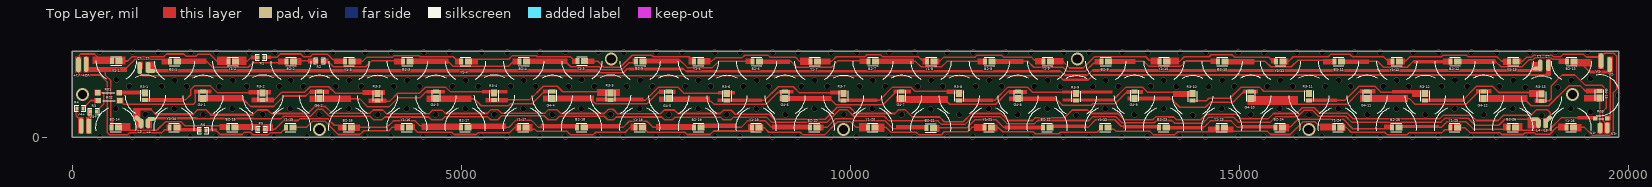
[diagram p0: Top Layer view]
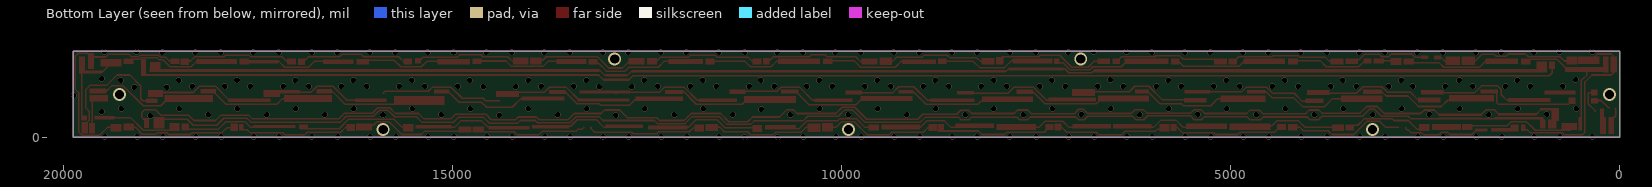
[diagram p1: Bottom Layer view, seen from below]
# Altium PCB MISC59163.PcbDoc
Units mil, origin at the board's own origin, x right, y up, seen from the top; angles counter-clockwise.
Board outline 19875 x 1102.36 mil, 2 copper layers (Top Layer, Bottom Layer); 87 components, 89 nets, 196 pads, 241 vias.

## Layer stack, top to bottom (the 12.6 mil dielectric is the usual default, probably not edited)
Top Solder: solder mask 0.4, Solder Resist, Dk 3.5
Top Layer: signal copper 1.4
Dielectric 1: dielectric 12.6, FR-4, Dk 4.8
Bottom Layer: signal copper 1.4
Bottom Solder: solder mask 0.4, Solder Resist, Dk 3.5

## Board outline
0,0 19875,0 19875,1102.36 0,1102.36

## Design rules (kind name [scope] priority, off if disabled: settings)
Clearance [All] p1: gap=0 ignorepadtopadclearanceinfootprint=TRUE
ComponentClearance [All] p1: gap=0 collisioncheckmode=3 verticalgap=0 showdistances=FALSE
HoleSize [All] p1: absolutevalues=TRUE maxlimit=1000 minlimit=1 maxpercent=80.000 minpercent=20.000
HoleToHoleClearance [All] p1: gap=0 allowstackedmicrovias=TRUE
MinimumSolderMaskSliver [All] p1: minsoldermaskwidth=0
PolygonConnect [All] p1: connectstyle=Relief reliefconductorwidth=10 reliefentries=4 polygonreliefangle="90 Angle" airgapwidth=10
RoutingVias [All] p1: holewidth=28 width=50 viastyle="Through Hole" minholewidth=3.94 minwidth=3.94 maxholewidth=1968.5 maxwidth=1968.5
SilkToSilkClearance [All] p1: silktosilkclearance=0
SilkToSolderMaskClearance [IsPad] p1: minsilkscreentomaskgap=0 clearancetoexposedcopper=TRUE
SolderMaskExpansion [All] p1: expansion=4 istentingtop=FALSE
Width [All] p1: maxlimit=100 minlimit=10 preferedwidth=20
24 further rules are at their usual default settings.

## Components (designator, comment, footprint, x,y, rotation, side; value= is the part's Value field where it differs from the comment)
B2-1 "2835A03-480B05-1S-F8" 2835LED带透镜 1299.21,930 r0 top locked
B2-2 "2835A03-480B05-1S-F8" 2835LED带透镜 2795.28,930 r0 top locked
B2-3 "2835A03-480B05-1S-F8" 2835LED带透镜 4291.34,930 r0 top locked
B2-4 "2835A03-480B05-1S-F8" 2835LED带透镜 5787.4,930 r0 top locked
B2-5 "2835A03-480B05-1S-F8" 2835LED带透镜 7283.46,930 r0 top locked
B2-6 "2835A03-480B05-1S-F8" 2835LED带透镜 8779.53,930 r0 top locked
B2-7 "2835A03-480B05-1S-F8" 2835LED带透镜 10275.59,930 r0 top locked
B2-8 "2835A03-480B05-1S-F8" 2835LED带透镜 11771.65,930 r0 top locked
B2-9 "2835A03-480B05-1S-F8" 2835LED带透镜 13267.72,930 r0 top locked
B2-10 "2835A03-480B05-1S-F8" 2835LED带透镜 14763.78,930 r0 top locked
B2-11 "2835A03-480B05-1S-F8" 2835LED带透镜 16259.84,930 r0 top locked
B2-12 "2835A03-480B05-1S-F8" 2835LED带透镜 17755.91,930 r0 top locked
B2-13 "2835A03-480B05-1S-F8" 2835LED带透镜 19251.97,930.71 r0 top locked
B2-14 "2835A03-480B05-1S-F8" 2835LED带透镜2 551.18,140 r0 top locked
B2-15 "2835A03-480B05-1S-F8" 2835LED带透镜2 2047.24,140 r0 top locked
B2-16 "2835A03-480B05-1S-F8" 2835LED带透镜2 3543.31,140 r0 top locked
B2-17 "2835A03-480B05-1S-F8" 2835LED带透镜2 5039.37,140 r0 top locked
B2-18 "2835A03-480B05-1S-F8" 2835LED带透镜2 6535.43,140 r0 top locked
B2-19 "2835A03-480B05-1S-F8" 2835LED带透镜2 8038.39,140 r0 top locked
B2-20 "2835A03-480B05-1S-F8" 2835LED带透镜2 9527.56,140 r0 top locked
B2-21 "2835A03-480B05-1S-F8" 2835LED带透镜2 11023.62,133.78 r0 top locked
B2-22 "2835A03-480B05-1S-F8" 2835LED带透镜2 12519.68,140 r0 top locked
B2-23 "2835A03-480B05-1S-F8" 2835LED带透镜2 14015.75,140 r0 top locked
B2-24 "2835A03-480B05-1S-F8" 2835LED带透镜2 15511.81,140 r0 top locked
B2-25 "2835A03-480B05-1S-F8" 2835LED带透镜2 17007.87,140 r0 top locked
B2-26 "2835A03-480B05-1S-F8" 2835LED带透镜2 18503.94,140 r0 top locked
G4-1 "2835A03-525G05-2P-F10" 2835LED带透镜3#1 1692.91,551.18 r0 top locked
G4-2 "2835A03-525G05-2P-F10" 2835LED带透镜3#1 3188.98,551.18 r0 top locked
G4-3 "2835A03-525G05-2P-F10" 2835LED带透镜3#1 4685.04,551.18 r0 top locked
G4-4 "2835A03-525G05-2P-F10" 2835LED带透镜3#1 6181.1,551.18 r0 top locked
G4-5 "2835A03-525G05-2P-F10" 2835LED带透镜3#1 7677.17,551.18 r0 top locked
G4-6 "2835A03-525G05-2P-F10" 2835LED带透镜3#1 9173.23,551.18 r0 top locked
G4-7 "2835A03-525G05-2P-F10" 2835LED带透镜3#1 10669.29,551.18 r0 top locked
G4-8 "2835A03-525G05-2P-F10" 2835LED带透镜3#1 12165.35,551.18 r0 top locked
G4-9 "2835A03-525G05-2P-F10" 2835LED带透镜3#1 13661.42,551.18 r0 top locked
G4-10 "2835A03-525G05-2P-F10" 2835LED带透镜3#1 15157.48,551.18 r0 top locked
G4-11 "2835A03-525G05-2P-F10" 2835LED带透镜3#1 16653.54,551.18 r0 top locked
G4-12 "2835A03-525G05-2P-F10" 2835LED带透镜3#1 18149.61,551.18 r0 top locked
G4-13 "2835A03-525G05-2P-F10" 2835LED带透镜2 19645.67,551.18 r270 top locked
R01 "jumper" 贴片跳线QM8.2-D01 465,570 r0 top
R1 "20Ω" R0805 2425,1025 r0 top value=20R
R02 "jumper" 贴片跳线QM8.2-D01 470,470 r0 top
R2 "20Ω" R0805 3180,980 r0 top value=20R
R03 "jumper" 贴片跳线 19575,240 r0 top
R3 "10Ω" R0805 275,330 r0 top value=10R
R3-1 "2835A03-630R05-2P-F10" 2835LED带透镜3#2 941.14,535.87 r0 top
R3-2 "2835A03-630R05-2P-F10" 2835LED带透镜3#2 2451.14,535.87 r0 top locked
R3-3 "2835A03-630R05-2P-F10" 2835LED带透镜3#2 3926.14,530.87 r0 top locked
R3-4 "2835A03-630R05-2P-F10" 2835LED带透镜3#2 5426.14,535.87 r0 top locked
R3-5 "2835A03-630R05-2P-F10" 2835LED带透镜3#2 6921.14,535.87 r0 top locked
R3-6 "2835A03-630R05-2P-F10" 2835LED带透镜3#2 8416.14,530.87 r0 top locked
R3-7 "2835A03-630R05-2P-F10" 2835LED带透镜3#2 9915,530 r0 top locked
R3-8 "2835A03-630R05-2P-F10" 2835LED带透镜3#2 11401.14,530.87 r0 top locked
R3-9 "2835A03-630R05-2P-F10" 2835LED带透镜3#2 12906.14,525.87 r0 top
R3-10 "2835A03-630R05-2P-F10" 2835LED带透镜3#2 14401.14,526.42 r0 top locked
R3-11 "2835A03-630R05-2P-F10" 2835LED带透镜3#2 15896.14,530.87 r0 top locked
R3-12 "2835A03-630R05-2P-F10" 2835LED带透镜3#2 17390,530 r0 top locked
R3-13 "2835A03-630R05-2P-F10" 2835LED带透镜3#2 18885,520 r0 top locked
R4 "10Ω" R0805 100,370 r0 top value=10R
R5 "20Ω" R0805 2435,100 r0 top value=20R
R6 "20Ω" R0805 1680,85 r0 top value=20R
Y1-1 "2835A03-585Y05-2P-F10" 2835LED带透镜1 551.18,935.71 r0 top
Y1-2 "2835A03-585Y05-2P-F10" 2835LED带透镜 2047.24,930 r0 top locked
Y1-3 "2835A03-585Y05-2P-F10" 2835LED带透镜 3543.31,930 r0 top locked
Y1-4 "2835A03-585Y05-2P-F10" 2835LED带透镜 5039.37,930 r0 top locked
Y1-5 "2835A03-585Y05-2P-F10" 2835LED带透镜 6535.43,935 r0 top locked
Y1-6 "2835A03-585Y05-2P-F10" 2835LED带透镜 8031.5,930 r0 top locked
Y1-7 "2835A03-585Y05-2P-F10" 2835LED带透镜 9527.56,930 r0 top locked
Y1-8 "2835A03-585Y05-2P-F10" 2835LED带透镜 11023.62,930 r0 top locked
Y1-9 "2835A03-585Y05-2P-F10" 2835LED带透镜 12519.68,930 r0 top locked
Y1-10 "2835A03-585Y05-2P-F10" 2835LED带透镜 14015.75,930 r0 top locked
Y1-11 "2835A03-585Y05-2P-F10" 2835LED带透镜 15511.81,930 r0 top locked
Y1-12 "2835A03-585Y05-2P-F10" 2835LED带透镜 17007.87,930 r0 top locked
Y1-13 "2835A03-585Y05-2P-F10" 2835LED带透镜 18503.94,930 r0 top locked
Y1-14 "2835A03-585Y05-2P-F10" 2835LED带透镜2 1299.21,140 r0 top locked
Y1-15 "2835A03-585Y05-2P-F10" 2835LED带透镜2 2795.28,140 r0 top locked
Y1-16 "2835A03-585Y05-2P-F10" 2835LED带透镜2 4291.34,140 r0 top locked
Y1-17 "2835A03-585Y05-2P-F10" 2835LED带透镜2 5787.4,140 r0 top locked
Y1-18 "2835A03-585Y05-2P-F10" 2835LED带透镜2 7283.46,140 r0 top locked
Y1-19 "2835A03-585Y05-2P-F10" 2835LED带透镜2 8779.53,140 r0 top locked
Y1-20 "2835A03-585Y05-2P-F10" 2835LED带透镜2 10275,140 r0 top locked
Y1-21 "2835A03-585Y05-2P-F10" 2835LED带透镜2 11771.65,140 r0 top locked
Y1-22 "2835A03-585Y05-2P-F10" 2835LED带透镜2 13267.72,140 r0 top locked
Y1-23 "2835A03-585Y05-2P-F10" 2835LED带透镜2 14763.78,140 r0 top locked
Y1-24 "2835A03-585Y05-2P-F10" 2835LED带透镜2 16259.84,140 r0 top locked
Y1-25 "2835A03-585Y05-2P-F10" 2835LED带透镜2 17755.91,140 r0 top locked
Y1-26 "2835A03-585Y05-2P-F10" 2835LED带透镜2 19251.97,140 r0 top locked

## Footprints (in the part's own frame and the unit in brackets; to place one, negate y for a bottom-side part, rotate by r counter-clockwise, add the part's x,y. Pads: shape width x height; smd on the part's side, far side on the other; paste and mask are expansions set on the pad)
2835LED带透镜 [mm]
  rect 1.3x2 smd: 1(-0.95,1.125)
  rect 2.3x2 smd: 2(1.35,1.125)
  silkscreen extent -6.2,-4.63 7.1,2.52
2835LED带透镜1 [mm]
  rect 1.3x2 smd: 1(-0.95,1.125)
  rect 2.3x2 smd: 2(1.35,1.125)
  silkscreen extent -6.2,-4.63 7.1,2.52
2835LED带透镜2 [mm]
  rect 1.3x2 smd: 1(-1.102,-0.35)
  rect 2.3x2 smd: 2(1.198,-0.35)
  silkscreen extent -6.35,-1.75 6.95,5.9
2835LED带透镜3#1 [mm]
  rect 2x1.3 smd: 1(-0.225,0.925)
  rect 2x2.3 smd: 2(-0.225,-1.375)
  silkscreen extent -6.87,-6.23 6.43,6.17
2835LED带透镜3#2 [mm]
  rect 2x1.3 smd: 1(-0.029,-1.433)
  rect 2x2.3 smd: 2(-0.029,0.867)
  silkscreen extent -6.62,-5.73 6.68,6.68
R0805 [mm]
  rect 1x1.27 smd: 1(-0.975,0.025) 2(1.025,0.025)
  silkscreen extent -1.85,-0.97 1.9,1.03
贴片跳线 [mm]
  rect 1.5x1.2 smd: 1(0,0) 2(4,0)
  silkscreen extent 1.14,0 2.79,0
贴片跳线QM8.2-D01 [mm]
  rect 1.8x1.7 smd: 1(-3.389,0.054) 2(3.611,0.054)
  silkscreen extent -1.92,0.05 2.14,0.05

## Part data
B2-1 B2-2 B2-3 B2-4 B2-5 B2-6 B2-7 B2-8 B2-9 B2-10 B2-11 B2-12 B2-13 B2-14 B2-15 B2-16 B2-17 B2-18 B2-19 B2-20 B2-21 B2-22 B2-23 B2-24 B2-25 B2-26 G4-1 G4-2 G4-3 G4-4 G4-5 G4-6 G4-7 G4-8 G4-9 G4-10 G4-11 G4-12 G4-13 R3-1 R3-2 R3-3 R3-4 R3-5 R3-6 R3-7 R3-8 R3-9 R3-10 R3-11 R3-12 R3-13 Y1-1 Y1-2 Y1-3 Y1-4 Y1-5 Y1-6 Y1-7 Y1-8 Y1-9 Y1-10 Y1-11 Y1-12 Y1-13 Y1-14 Y1-15 Y1-16 Y1-17 Y1-18 Y1-19 Y1-20 Y1-21 Y1-22 Y1-23 Y1-24 Y1-25 Y1-26: library part LED2
R01 R02: library part Res2, "QM8.2-D01  silver"
R1 R2 R3 R4 R5 R6: library part Res2, "0805 chip resistor"
R03: library part Res2, "QM52-D01  silver"

## Free pads (board coordinates)
  oval 59.06x196.85 smd: 0(82.68,933.07) 0(118.11,145) 0(181.1,937.01) 0(216.54,145) 0(19650,981.4) 0(19760,932.77)
  oval 59.06x118.11 smd rot 45: 0(853.35,229.84)
  oval 59.06x157.48 smd: 0(870,890)
  oval 59.06x129.92 smd: 0(885.83,177.68) 0(975,180) 0(18846.73,177.52) 0(18938.03,177.52)
  oval 59.06x147.64 smd: 0(978.03,896.18) 0(18867.44,925.7)
  oval 118.11x51.18 smd: 0(1012.52,850.91) 0(18832.95,880.43)
  oval 102.36x47.24 smd: 0(1016.34,235.12) 0(18805.39,232.64)
  oval 59.06x118.11 smd rot 135: 0(18970.51,229.68)
  oval 59.06x149.61 smd: 0(18973.74,923.74)
  oval 59.05x141.73 smd: 0(19640,120)
  oval 59.06x141.73 smd: 0(19730,120)

## Via types
v1: diameter 70.87, hole 70.87, Top Layer to Bottom Layer, 234 vias
v2: diameter 165.35, hole 118.11, Top Layer to Bottom Layer, 7 vias

## Nets (pads, with @x,y where several pads share a name; then routed paths per layer and width w, separated by ;. In a path a pad name is that pad's centre, name@x,y a point inside that pad or via, vN(x,y) a via of type N, cw(c..) or ccw(c..) an arc to the next point about the centre after c; other vN are vias at no path point)
NetB2-1_2: B2-1.2 B2-2.1 | length 1469.4
  Top Layer w20: B2-1.2@1352.36,980 1725,980 1805,900 2265,900 2325,960 2743.58,960 B2-2.1
NetB2-2_2: B2-2.2 R2.1 | length 296
  Top Layer w20: B2-2.2 2855.12,980.98 R2.1
NetB2-3_1: B2-3.1 R2.2 | length 1102.6
  Top Layer w20: R2.2 3284.02,980.98 3360,905 3775,905 3855,985 4243.23,985 B2-3.1
NetB2-3_2: B2-3.2 B2-4.1 | length 1458.8
  Top Layer w20: B2-3.2 4835.71,974.29 4900,910 5605,910 5669.29,974.29 B2-4.1
NetB2-4_2: B2-4.2 B2-5.1 | length 1496.1
  Top Layer w20: B2-4.2 5864.84,950 6365,950 6410,905 6775,905 6815,865 7065,865 7160,960 7231.77,960 B2-5.1
NetB2-5_2: B2-5.2 B2-6.1 | length 1484.8
  Top Layer w20: B2-5.2 7352.32,990 7815,990 7910,895 8230,895 8310,975 8741.42,975 B2-6.1
NetB2-6_2: B2-6.2 B2-7.1 | length 1475.9
  Top Layer w20: B2-6.2 9240.71,974.29 9315,900 9760,900 9845,985 10227.48,985 B2-7.1
NetB2-7_2: B2-7.2 B2-8.1 | length 1462.9
  Top Layer w20: B2-7.2 10840.71,974.29 10910,905 11175,905 11244.29,974.29 B2-8.1
NetB2-8_2: B2-8.2 B2-9.1 | length 1508.5
  Top Layer w20: B2-8.2 12285.71,974.29 12360,900 12735,900 12785,850 13025,850 13123.79,948.79 13204.81,948.79 B2-9.1
NetB2-9_2: B2-9.2 B2-10.1 | length 1463.5
  Top Layer w20: B2-9.2 13775.71,974.29 13840,910 14245,910 14315,980 14720.67,980 B2-10.1
NetB2-10_2: B2-10.2 B2-11.1 | length 1476
  Top Layer w20: B2-10.2 15335.71,974.29 15405,905 15670,905 15755,990 16206.85,990 16222.44,974.41 B2-11.1
NetB2-11_2: B2-11.2 B2-12.1 | length 1467.1
  Top Layer w20: B2-11.2 16780.71,974.29 16855,900 17160,900 17234.29,974.29 B2-12.1
NetB2-12_2: B2-12.2 B2-13.1 | length 1500.5
  Top Layer w20: B2-12.2 18295.71,974.29 18365,905 18635,905 18725,995 18775,995 18800,1020 19010,1020 19030,1000 19145,1000 19170,975 B2-13.1
NetB2-14_2: B2-14.2 B2-15.1 | length 1498.5
  Top Layer w20: B2-14.2 604.25,126.22 640.47,90 1090,90 1200,200 1400,200 1455,145 1988.27,145 2003.86,129.41 B2-15.1
NetB2-15_2: B2-15.2 R5.1 | length 315.8
  Top Layer w20: B2-15.2 2376.69,126.22 2396.61,106.3 R5.1
NetB2-16_1: B2-16.1 R5.2 | length 1132.5
  Top Layer w20: R5.2 2605.98,100.98 2720,215 2905,215 2925,235 3290,235 3370.66,154.34 3484.33,154.34 3499.92,138.75 B2-16.1
NetB2-16_2: B2-16.2 B2-17.1 | length 1474.9
  Top Layer w20: B2-16.2 4046.22,126.22 4130,210 4410,210 4471.72,148.28 4973.92,148.28 B2-17.1
NetB2-17_2: B2-17.2 B2-18.1 | length 1483.2
  Top Layer w20: B2-17.2 5611.22,126.22 5705,220 5900,220 5993.78,126.22 B2-18.1
NetB2-18_2: B2-18.2 B2-19.1 | length 1477.7
  Top Layer w20: B2-18.2 7081.22,126.22 7160,205 7390,205 7468.78,126.22 B2-19.1
NetB2-19_2: B2-19.2 B2-20.1 | length 1468
  Top Layer w20: B2-19.2 8596.22,126.22 8680,210 8910,210 8993.78,126.22 B2-20.1
NetB2-20_2: B2-20.2 B2-21.1 | length 1506.5
  Top Layer w20: B2-20.2 9701.22,126.22 9810,235 10030,235 10055,210 10450,210 10550,110 10970.24,110 B2-21.1
NetB2-21_2: B2-21.2 B2-22.1 | length 1489.9
  Top Layer w20: B2-21.2 11500,120 11605,225 11875,225 11973.78,126.22 B2-22.1
NetB2-22_2: B2-22.2 B2-23.1 | length 1487.3
  Top Layer w20: B2-22.2 13056.22,126.22 13155,225 13400,225 13485,140 13958.58,140 B2-23.1
NetB2-23_2: B2-23.2 B2-24.1 | length 1474.9
  Top Layer w20: B2-23.2 14070.41,133.71 14553.71,133.71 14630,210 14895,210 14978.78,126.22 B2-24.1
NetB2-24_2: B2-24.2 B2-25.1 | length 1505.3
  Top Layer w20: B2-24.2 15566.04,133.28 15658.28,133.28 15755,230 16340,230 16460,110 16948.9,110 16964.49,125.59 B2-25.1
NetB2-25_2: B2-25.2 B2-26.1 | length 1489.2
  Top Layer w20: B2-25.2 17596.22,126.22 17670,200 17915,200 18010,105 18444.96,105 18460.55,120.59 B2-26.1 B2-26.1@18459.33,125
NetB2-26_2: B2-26.2 R03.1 | length 1008.7
  Top Layer w20: B2-26.2 18557.01,126.22 18593.23,90 18980,90 19142.5,252.5 19477.5,252.5
NetG4-1_1: G4-1.1 R02.2 | length 1222.7
  Top Layer w20: R02.2 R02.2@614.12,472.12 ; R02.2@615.62,467.5 618.74,467.5 661.24,425 1560,425 1585,450 1585,565 1607.6,587.6 G4-1.1
NetG4-1_2: G4-1.2 G4-2.1 | length 1618.1
  Top Layer w20: G4-1.2 1704.39,476.72 2213.28,476.72 2295,395 2590,395 2725,530 3005,530 3057.46,582.46 3174.98,582.46 G4-2.1
NetG4-2_2: G4-2.2 G4-3.1 | length 1622.3
  Top Layer w20: G4-2.2 3692.95,497.05 3800,390 4075,390 4190,505 4470,505 4550,585 4673.58,585 G4-3.1
NetG4-3_2: G4-3.2 G4-4.1 | length 1609.8
  Top Layer w20: G4-3.2 5167.95,497.05 5260,405 5610,405 5635,430 5910,430 6067.6,587.6 G4-4.1
NetG4-4_2: G4-4.2 G4-5.1 | length 1595
  Top Layer w20: G4-4.2 6672.95,497.05 6700,470 6700,460 6730,430 7390,430 7547.6,587.6 G4-5.1
NetG4-5_2: G4-5.2 G4-6.1 | length 1593.8
  Top Layer w20: G4-5.2 7700.35,465 8210,465 8250.69,424.31 8919.31,424.31 9070,575 9151.77,575 G4-6.1
NetG4-6_2: G4-6.2 G4-7.1 | length 1600.3
  Top Layer w20: G4-6.2 9186.42,475 9760,475 9815,420 10425,420 10570,565 10570,570 10587.6,587.6 G4-7.1
NetG4-7_2: G4-7.2 G4-8.1 | length 1596.7
  Top Layer w20: G4-7.2 10660.43,491.14 10701.57,450 11255,450 11280,425 11870,425 12032.6,587.6 G4-8.1
NetG4-8_2: G4-8.2 G4-9.1 | length 1605.7
  Top Layer w20: G4-8.2 12642.95,497.05 12730,410 13097.5,410 13117.5,430 13405,430 13562.6,587.6 G4-9.1
NetG4-9_2: G4-9.2 G4-10.1 | length 1626.4
  Top Layer w20: G4-9.2 14122.95,497.05 14235,385 14565,385 14630,450 14920,450 15057.6,587.6 G4-10.1
NetG4-10_2: G4-10.2 G4-11.1 | length 1593.3
  Top Layer w20: G4-10.2 15672.95,497.05 15745,425 16385,425 16547.6,587.6 G4-11.1
NetG4-11_2: G4-11.2 G4-12.1 | length 1593.3
  Top Layer w20: G4-11.2 17187.95,497.05 17260,425 17915,425 18077.6,587.6 G4-12.1
NetG4-12_2: G4-12.2 G4-13.1 | length 1672.4
  Top Layer w20: G4-12.2 18140.75,492.89 18170.12,463.52 18695,463.52 18753.52,405 18980,405 19235,660 19385,660 19460,585 19622.32,585 G4-13.1
NetR1_1: R1.1 Y1-2.2 | length 307.6
  Top Layer w20: Y1-2.2 2249.29,974.29 2300.98,1025.98 R1.1
NetR01_1: R01.1 R3.2 | length 351.9
  Top Layer w20: R3.2 315.35,336.3 410,430.95 410,560.4 398.28,572.12 R01.1
NetR1_2: R1.2 Y1-3.1 | length 1126.3
  Top Layer w20: R1.2 2630.98,1025.98 2675,1070 2940,1070 2975,1035 3060,1035 3090,1065 3285,1065 3355,995 3490.32,995 3505.91,979.41 Y1-3.1
NetR01_2: R01.2 R3-1.2 | length 335.3
  Top Layer w20: R01.2 622.62,587.6 R3-1.2@936.02,587.6
NetR02_1: R02.1 R4.2 | length 241.2
  Top Layer w20: R4.2 140.35,376.3 150.04,385.98 155.35,385.98 241.49,472.12 R02.1
NetR3-1_1: R3-1.1 R3-2.2 | length 1684.3
  Top Layer w20: R3-1.1 1459.45,479.45 1525,545 1525,615 1570,660 1780,660 1870,570 R3-2.2 ; 2310,600 2325,585
NetR3-2_1: R3-2.1 R3-3.2 | length 1580.9
  Top Layer w20: R3-2.1 2594.45,479.45 2695,580 2990,580 3060,650 3300,650 3385,565 R3-3.2
NetR3-3_1: R3-3.1 R3-4.2 | length 1605.4
  Top Layer w20: R3-3.1 3934.45,465 4085,465 4185,565 4465,565 4540,640 4805,640 4862.5,582.5 5412.5,582.5 R3-4.2
NetR3-4_1: R3-4.1 R3-5.2 | length 1602.9
  Top Layer w20: R3-4.1 5879.45,479.45 6055,655 6235,655 6305,585 6850,585 6865,570 R3-5.2
NetR3-5_1: R3-5.1 R3-6.2 | length 1600.4
  Top Layer w20: R3-5.1 6924.45,475 7370,475 7540,645 7785,645 7865,565 R3-6.2
NetR3-6_1: R3-6.1 R3-7.2 | length 1607.1
  Top Layer w20: R3-6.1 8899.45,474.45 9075,650 9270,650 9350,570 9907.99,570 R3-7.2
NetR3-7_1: R3-7.1 R3-8.2 | length 1590.3
  Top Layer w20: R3-7.1 10373.58,473.58 10545,645 10780,645 10835,590 11375,590 R3-8.2
NetR3-8_1: R3-8.1 R3-9.2 | length 1610.9
  Top Layer w20: R3-8.1 11859.45,474.45 12030,645 12275,645 12340,580 12885,580 R3-9.2
NetR3-9_1: R3-9.1 R3-10.2 | length 1607.1
  Top Layer w20: R3-9.1 13369.45,469.45 13545,645 13755,645 13820,580 14370,580 R3-10.2@14400,550
NetR3-10_1: R3-10.1 R3-11.2 | length 1600.6
  Top Layer w20: R3-10.1 14580,470 14610,500 14880,500 15025,645 15260,645 15315,590 15870,590 R3-11.2
NetR3-11_1: R3-11.1 R3-12.2 | length 1606.3
  Top Layer w20: R3-11.1 16359.45,474.45 16540,655 16745,655 16820,580 17372.99,580 R3-12.2
NetR3-12_1: R3-12.1 R3-13.2 | length 1613.6
  Top Layer w20: R3-12.1 17868.58,473.58 18050,655 18255,655 18335,575 18880,575 R3-13.2@18890,585
NetR6_1: R6.1 Y1-14.2 | length 311.9
  Top Layer w20: Y1-14.2 1352.28,126.22 1392.52,85.98 R6.1
NetR6_2: R6.2 Y1-15.1 | length 1127.5
  Top Layer w20: R6.2 1854.02,85.98 1905,35 2185,35 2215,65 2295,65 2330,30 2520,30 2550,60 2685.67,60 2722.52,96.85 2736.3,96.85 2751.89,112.44 Y1-15.1
NetY1-1_2: Y1-1.2 Y1-2.1 | length 1503.1
  Top Layer w20: Y1-1.2 715,980 770,1035 1180,1035 1215,1070 1435,1070 1465,1040 1590,1040 1615,1065 1775,1065 1865.71,974.29 Y1-2.1
NetY1-3_2: Y1-3.2 Y1-4.1 | length 1468.2
  Top Layer w20: Y1-3.2 3734.29,974.29 3790,1030 4120,1030 4140,1050 4460,1050 4475,1035 4900,1035 4960.71,974.29 Y1-4.1
NetY1-4_2: Y1-4.2 Y1-5.1 | length 1466.2
  Top Layer w20: Y1-4.2 5121.89,1003.66 5613.66,1003.66 5660,1050 5965,1050 5980,1035 6405,1035 6460.71,979.29 Y1-5.1
NetY1-5_2: Y1-5.2 Y1-6.1 | length 1544.1
  Top Layer w20: Y1-5.2 6755.71,979.29 6835,900 7045,900 7200,1055 7450,1055 7470,1035 7933.39,1035 7964.72,1003.66 7978.5,1003.66 7994.09,988.07 Y1-6.1
NetY1-6_2: Y1-6.2 Y1-7.1 | length 1472.4
  Top Layer w20: Y1-6.2 8219.29,974.29 8265,1020 8610,1020 8645,1055 8945,1055 8970,1030 9295,1030 9350,975 9489.45,975 Y1-7.1
NetY1-7_2: Y1-7.2 Y1-8.1 | length 1476.5
  Top Layer w20: Y1-7.2 9759.29,974.29 9820,1035 10190,1035 10215,1060 10390,1060 10415,1035 10880,1035 10926.93,988.07 10972.44,988.07 Y1-8.1
NetY1-8_2: Y1-8.2 Y1-9.1 | length 1472.4
  Top Layer w20: Y1-8.2 11149.29,974.29 11205,1030 11605,1030 11630,1055 11945,1055 11970,1030 12330,1030 12370,990 12466.69,990 12482.28,974.41 Y1-9.1
NetY1-9_2: Y1-9.2 Y1-10.1 | length 1525.7
  Top Layer w20: Y1-9.2 12735.71,974.29 12820,890 12995,890 13140,1035 13800,1035 13845,990 13962.76,990 13978.35,974.41 Y1-10.1
NetY1-10_2: Y1-10.2 Y1-11.1 | length 1476.6
  Top Layer w20: Y1-10.2 14234.29,974.29 14295,1035 14615,1035 14640,1060 14905,1060 14935,1030 15380,1030 15420,990 15458.82,990 15474.41,974.41 Y1-11.1
NetY1-11_2: Y1-11.2 Y1-12.1 | length 1480.7
  Top Layer w20: Y1-11.2 15634.29,974.29 15695,1035 16145,1035 16175,1065 16425,1065 16434.97,1055.03 16455,1035 16855,1035 16915.71,974.29 Y1-12.1
NetY1-12_2: Y1-12.2 Y1-13.1 | length 1472.4
  Top Layer w20: Y1-12.2 17134.29,974.29 17195,1035 17600,1035 17620,1055 17920,1055 17940,1035 18315,1035 18370,980 18460.83,980 Y1-13.1
NetY1-15_2: Y1-15.2 Y1-16.1 | length 1546.3
  Top Layer w20: Y1-15.2 3011.22,126.22 3090,205 3250,205 3420,35 3700,35 3750,85 4070,85 4111.22,126.22 Y1-16.1
NetY1-16_2: Y1-16.2 Y1-17.1 | length 1481.1
  Top Layer w20: Y1-16.2 4361.79,102.94 4402.06,102.94 4440,65 4880,65 4910,35 5195,35 5220,60 5625,60 5691.22,126.22 Y1-17.1
NetY1-17_2: Y1-17.2 Y1-18.1 | length 1485.2
  Top Layer w20: Y1-17.2 5855.79,105 5945,105 5975,75 6365,75 6410,30 6695,30 6730,65 7110,65 7171.22,126.22 Y1-18.1
NetY1-18_2: Y1-18.2 Y1-19.1 | length 1489.2
  Top Layer w20: Y1-18.2 7336.54,126.22 7397.76,65 7875,65 7905,35 8200,35 8245,80 8703.7,80 8720.55,96.85 8736.14,112.44 Y1-19.1
NetY1-19_2: Y1-19.2 Y1-20.1 | length 1545.8
  Top Layer w20: Y1-19.2 8832.91,120 8900,120 8955,65 9360,65 9395,30 9670,30 9840,200 10005,200 10078.78,126.22 Y1-20.1
NetY1-20_2: Y1-20.2 Y1-21.1 | length 1485.8
  Top Layer w20: Y1-20.2 10463.78,126.22 10525,65 10850,65 10885,30 11170,30 11210,70 11510,70 11566.22,126.22 Y1-21.1
NetY1-21_2: Y1-21.2 Y1-22.1 | length 1480.9
  Top Layer w20: Y1-21.2 11825.04,120 11910,120 11960,70 12355,70 12380,45 12680,45 12700,65 13176.89,65 13224.33,112.44 Y1-22.1
NetY1-22_2: Y1-22.2 Y1-23.1 | length 1431.5
  Top Layer w20: Y1-22.2 13336.1,105 13390,105 13420,75 13855,75 13900,30 14170,30 14210,70 14647.5,70 14677.5,100
NetY1-23_2: Y1-23.2 Y1-24.1 | length 1542.2
  Top Layer w20: Y1-23.2 14840.32,96.85 14898.15,96.85 14920,75 15365,75 15405,35 15655,35 15820,200 15975,200 16021.72,153.28 16189.39,153.28 Y1-24.1
NetY1-24_2: Y1-24.2 Y1-25.1 | length 1493.3
  Top Layer w20: Y1-24.2 16378.78,126.22 16440,65 16870,65 16905,30 17155,30 17185,60 17605,60 17641.85,96.85 17696.93,96.85 17712.52,112.44 Y1-25.1
NetY1-25_2: Y1-25.2 Y1-26.1 | length 1497.6
  Top Layer w20: Y1-25.2 17805.92,123.37 17901.63,123.37 17965,60 18350,60 18375,35 18650,35 18675,60 18795,60 18815,40 18990,40 19076.22,126.22 Y1-26.1
V1+: pad.0@82.68,933.07 Y1-1.1 Y1-14.1 | length 2632.3
  Top Layer w20: Y1-1.1 513.78,993.78 498.19,1009.37 350.63,1009.37 290,1070 110,1070 90.15,1050.15 90.15,940.54 82.68,933.07 86.34,929.4 86.34,823.66 110,800 360,800 450,710 450,65 485,30 710,30 740,60 1155,60 1191.85,96.85 1240.24,96.85 1255.83,112.44 Y1-14.1
V1-: pad.0@19650,981.4 Y1-13.2 Y1-26.2 | length 3024.2
  Top Layer w20: Y1-13.2 18639.29,974.29 18695,1030 18760,1030 18785,1055 19020,1055 19040,1035 19130,1035 19160,1065 19425,1065 19460,1030 19631.96,1030 pad.0@19650,1011.96 ; Y1-26.2 19438.78,126.22 19540,25 19765,25 19810,70 19810,575 19850,615 19850,1045 19815,1080 19696.67,1080 19650,1033.33 pad.0@19650,1011.96 ; pad.0@19650,975 19650,981.4 pad.0@19650,1011.96
V2+: B2-1.1 B2-14.1 pad.0@181.1,937.01 | length 2036.8
  Top Layer w20: pad.0@181.1,937.01 181.1,913.04 229.14,865 425,865 670,865 805,1000 1165,1000 1185,980 B2-1.1@1261.81,980 ; pad.0@187.76,907.24 187.76,875.29 199.14,863.91 221.09,863.91 ; 425,870 425,800 500,725 500,134.01 B2-14.1
V2-: B2-13.2 pad.0@19760,932.77 R03.2 | length 1320.7
  Top Layer w20: B2-13.2 19370,975 19514.69,830.31 19735,830.31 19760,855.31 19760,922.77 19760,932.77 19760,888.04 19770,878.04 19767.47,875.51 19767.47,265.34 19755.76,253.62 19746.1,253.62 R03.2
V3+: pad.0@216.54,145 R3.1 | length 194.3
  Top Layer w20: pad.0@216.54,145 216.54,305.59 236.61,325.67 R3.1
V3-: pad.0@19730,120 R3-13.1 | length 1678.1
  Top Layer w20: R3-13.1 18890.28,470 18985,470 19010,495 19010,660 19150,800 19315,800 19445,670 19660,670 19715,615 19715,375 19675,335 19675,215 19730,160 pad.0@19730,120
V4+: pad.0@118.11,145 R4.1 | length 254.9
  Top Layer w20: R4.1 55,364.37 55,277.01 118.11,213.9 pad.0@118.11,145
V4-: G4-13.2 pad.0@19640,120 | length 387.4
  Top Layer w20: G4-13.2 19631.89,180.02 19640,171.91 pad.0@19640,120
copper on no net: | length 74818.7
  Top Layer w20: 853.35,229.84 832.47,250.72 832.47,322.47 865,355 1015,355 1080,290 1320,290 1555,290 1555,300 ; 871.73,905.28 871.73,828.49 910.22,790 12685,790 12740,735 12900,735 13060,735 13120,795 18925,795 18966.26,836.26 18966.26,935.24 18970.24,939.21 ; 1012.52,865.91 1018.49,859.94 1068.35,859.94 1087.01,841.29 6778.71,841.29 6790,830 7085,830 7135,880 7855,880 7885,850 12700,850 12755,795 12900,795 13045,795 13120,870 13435,870 13443.79,861.21 14991.29,861.21 15000.07,870 18780.61,870 18790.61,880 18813.08,880 ; 1016.34,235.12 2685.12,235.12 2720,270 3065,270 3155,360 3220,360 3310,270 3830,270 3875,225 3985,225 4020,260 4585,260 4620,225 4755,225 4795,265 5340,265 5380,225 5470,225 5520,275 6070,275 6120,225 6220,225 6265,270 6840,270 6885,225 6960,225 6995,260 7580,260 7615,225 7715,225 7745,255 8340,255 8370,225 8465,225 8495,255 8930,255 8995,190 9700,190 9865,355 9960,355 10045,270 10440,270 10500,210 11130,210 11175,165 11475,165 11575,265 11925,265 12015,175 12370,175 12410,215 13070,215 13120,265 13415,265 13495,185 13910,185 13940,215 14135,215 14170,180 14530,180 14605,255 14930,255 14995,190 15395,190 15467.5,262.5 15747.5,262.5 15830,345 15945,345 16020,270 16370,270 16445,195 17595,195 17645,245 17945,245 18035,155 18335,155 18412.64,232.64 18805.39,232.64 ; 1320,295 1555,295 1555,300 ; 18970.51,229.68 18995,254.17 18995,320 18960,355 18825,355 18755,285 18400,285 18330,215 18050,215 17985,280 17620,280 17575,235 16465,235 16390.76,309.24 16035.76,309.24 15965,380 15810,380 15735,305 15440,305 15370,235 15025,235 14965,295 14575,295 14505,225 14195,225 14160,260 13925,260 13890,225 13520,225 13440,305 13095,305 13050,350 12855,350 12755,250 12380,250 12345,215 12025,215 11935,305 11560,305 11455,200 11210,200 11150,260 10800,260 10705,355 10625,355 10575,305 10075,305 9995,385 9835,385 9680,230 9025,230 8960,295 8525,295 8473.28,346.72 8371.72,346.72 8330,305 7785,305 7740,350 7610,350 7560,300 7015,300 6955,360 6895,360 6840,305 6280,305 6230,355 6125,355 6080,310 5515,310 5470,355 5385,355 5335,305 4800,305 4760,345 4630,345 4585,300 4045,300 3995,350 3870,350 3830,310 3340,310 3255,395 3120,395 3030,305 2797.5,305 2560,305 2515,350 2385,350 2320,285 1790,285 1720,355 1615,355 1560,300 1555,300
  other v1: 10825.67,-1.06 11245.04,-1.06 353.23,5.16 772.6,5.16 1101.26,5.16 1520.63,5.16 1849.29,5.16 2268.66,5.16 2597.32,5.16 3016.69,5.16 3345.35,5.16 3764.73,5.16 4093.38,5.16 4512.76,5.16 4841.41,5.16 5260.79,5.16 5589.45,5.16 6008.82,5.16 6337.48,5.16 6756.85,5.16 7085.51,5.16 7504.88,5.16 7840.43,5.16 8259.81,5.16 8581.57,5.16 9000.95,5.16 9329.6,5.16 9748.98,5.16 10077.04,5.16 10496.42,5.16 11573.7,5.16 11993.07,5.16 12321.73,5.16 12741.1,5.16 13069.76,5.16 13489.14,5.16 13817.79,5.16 14237.17,5.16 14565.82,5.16 14985.2,5.16 15313.86,5.16 15733.23,5.16 16061.89,5.16 16481.26,5.16 16809.92,5.16 17229.29,5.16 17557.95,5.16 17977.32,5.16 18305.98,5.16 18725.36,5.16 19054.01,5.16 19473.39,5.16 18886.14,279.17 12907.28,285.04 14402.28,285.59 9916.14,289.17 17391.14,289.17 1684.06,290.35 3180.12,290.35 3927.28,290.04 4676.18,290.35 6172.24,290.35 7668.31,290.35 8417.28,290.04 9164.37,290.35 10660.43,290.35 11402.28,290.04 12156.5,290.35 13652.56,290.35 15148.62,290.35 15897.28,290.04 16644.69,290.35 18140.75,290.35 942.28,295.04 2452.28,295.04 5427.28,295.04 6922.28,295.04 19510.83,329.76 11035.35,362.13 562.91,368.35 1310.94,368.35 2058.98,368.35 2807.01,368.35 3555.04,368.35 4303.07,368.35 5051.1,368.35 5799.13,368.35 6547.16,368.35 7295.2,368.35 8050.12,368.35 8791.26,368.35 9539.29,368.35 10286.73,368.35 11783.39,368.35 12531.42,368.35 13279.45,368.35 14027.48,368.35 14775.51,368.35 15523.54,368.35 16271.57,368.35 17019.61,368.35 17767.64,368.35 18515.67,368.35 19263.7,368.35 19874.02,539.45 18676.45,642.36 19095.83,642.36 12697.6,648.23 13116.97,648.23 14192.6,648.78 14611.97,648.78 9706.45,652.36 10125.83,652.36 17181.45,652.36 17600.83,652.36 3717.6,653.23 4136.97,653.23 8207.6,653.23 8626.97,653.23 11192.6,653.23 11611.97,653.23 15687.6,653.23 16106.97,653.23 1474.37,653.54 1893.74,653.54 2970.43,653.54 3389.81,653.54 4466.49,653.54 4885.87,653.54 5962.56,653.54 6381.93,653.54 7458.62,653.54 7877.99,653.54 8954.68,653.54 9374.06,653.54 10450.75,653.54 10870.12,653.54 11946.81,653.54 12366.18,653.54 13442.87,653.54 13862.25,653.54 14938.94,653.54 15358.31,653.54 16435,653.54 16854.37,653.54 17931.06,653.54 18350.44,653.54 732.6,658.23 1151.97,658.23 2242.6,658.23 2661.97,658.23 5217.6,658.23 5636.97,658.23 6712.6,658.23 7131.97,658.23 1316.93,732.17 2064.96,732.17 2812.99,732.17 3561.02,732.17 4309.06,732.17 5057.09,732.17 5805.12,732.17 7301.18,732.17 8049.21,732.17 8797.24,732.17 9545.28,732.17 10293.31,732.17 11041.34,732.17 11789.37,732.17 12537.4,732.17 13285.43,732.17 14033.46,732.17 14781.5,732.17 15529.53,732.17 16277.56,732.17 17025.59,732.17 17773.62,732.17 18521.65,732.17 19269.69,732.87 6553.15,737.17 568.9,737.87 19510.83,749.14 1107.24,1095.35 1526.62,1095.35 1855.27,1095.35 2274.65,1095.35 2603.31,1095.35 3022.68,1095.35 3351.34,1095.35 3770.71,1095.35 4099.37,1095.35 4518.74,1095.35 4847.4,1095.35 5266.77,1095.35 5595.43,1095.35 6014.81,1095.35 7091.49,1095.35 7510.87,1095.35 7839.53,1095.35 8258.9,1095.35 8587.56,1095.35 9006.93,1095.35 9335.59,1095.35 9754.96,1095.35 10083.62,1095.35 10502.99,1095.35 10831.65,1095.35 11251.03,1095.35 11579.68,1095.35 11999.06,1095.35 12327.71,1095.35 12747.09,1095.35 13075.75,1095.35 13495.12,1095.35 13823.78,1095.35 14243.15,1095.35 14571.81,1095.35 14991.18,1095.35 15319.84,1095.35 15739.22,1095.35 16067.87,1095.35 16487.25,1095.35 16815.9,1095.35 17235.28,1095.35 17563.94,1095.35 17983.31,1095.35 18311.97,1095.35 18731.34,1095.35 19060,1096.06 19479.37,1096.06 6343.46,1100.35 6762.84,1100.35 359.21,1101.06 778.59,1101.06
  other v2: 3180,98.43 9915,98.43 15895,98.43 133.86,551.18 19285,551.18 6930,1003.94 12920,1003.94

## Keep-outs
Keep-Out Layer:
  the board outline again, w10

## Other copper
Top Layer:
  rectangle net V1+: 265,940 545,1035
  rectangle net NetY1-1_2: 555,935 685,1035
  rectangle net NetR3-1_1: 895,450 1440,505
  rectangle net NetR3-8_1: 11350,450 11835,500
  rectangle net NetR3-7_1: 11240,555 11445,615
  rectangle: 13115,840 18900,875
  rectangle net NetR3-12_1: 18725,520 18920,605
  rectangle net NetR3-12_1: 17345,450 17890,495
  rectangle net NetG4-12_2: 18080,453.52 18705,545
  rectangle net NetR3-11_1: 17220,520 17430,605
  rectangle net NetR3-11_1: 16965,560 17430,605
  rectangle net NetR3-9_1: 14150,515 14445,595
  rectangle: 945,830 6765,875
  rectangle net NetR3-6_1: 9740,550 9955,600
  rectangle net NetG4-12_2: 19460,565 19670,625
  rectangle net V4-: 19430,460 19670,545
  rectangle: 2590,305 3005,320
  rectangle net V2-: 19700,215 19780,280
  rectangle net NetB2-26_2: 19350,230 19605,275
  rectangle net V1-: 19255,75 19400,170
  rectangle net NetY1-25_2: 19100,85 19235,175
  rectangle: 18905,120 18970,245
  rectangle: 18705,110 18845,260
  rectangle net NetB2-26_2: 18510,80 18640,180
  rectangle net NetB2-25_2: 18390,85 18485,175
  rectangle net NetY1-25_2: 17760,80 17860,175
  rectangle net NetY1-24_2: 17690,85 17745,170
  rectangle net NetB2-25_2: 17020,120 17570,160
  rectangle net NetB2-24_2: 16860,105 16975,165
  rectangle net NetY1-24_2: 16260,80 16365,170
  rectangle net NetY1-23_2: 16040,85 16245,175
  rectangle net NetB2-24_2: 15505,75 15640,170
  rectangle net NetB2-23_2: 15015,110 15480,160
  rectangle net NetY1-23_2: 14760,60 14925,140
  rectangle net NetY1-22_2: 14600,60 14745,140
  rectangle net NetB2-23_2: 14015,100 14540,145
  rectangle net NetB2-22_2: 13510,110 13980,155
  rectangle net NetB2-22_2: 12555,120 13040,165
  rectangle net NetB2-21_2: 11985,100 12490,150
  rectangle net NetY1-21_2: 11775,75 11895,165
  rectangle net NetY1-20_2: 11595,80 11755,170
  rectangle net NetB2-21_2: 11025,70 11150,160
  rectangle net NetB2-20_2: 10590,100 10985,160
  rectangle net NetY1-20_2: 10275,70 10440,175
  rectangle net NetY1-19_2: 10115,75 10255,180
  rectangle net NetB2-20_2: 9525,85 9655,165
  rectangle net NetB2-19_2: 8995,100 9490,165
  rectangle net NetY1-19_2: 8780,80 8885,170
  rectangle net NetY1-18_2: 8690,70 8770,170
  rectangle net NetB2-19_2: 8045,120 8540,175
  rectangle net NetB2-18_2: 7505,95 8015,170
  rectangle net NetY1-18_2: 7280,90 7385,170
  rectangle net NetY1-17_2: 7180,85 7265,175
  rectangle net NetB2-18_2: 6540,110 7035,170
  rectangle net NetB2-17_2: 6020,110 6515,170
  rectangle net NetY1-17_2: 5790,75 5915,170
  rectangle net NetY1-16_2: 5700,80 5775,170
  rectangle net NetB2-17_2: 5050,105 5580,175
  rectangle net NetB2-16_2: 4490,90 5015,175
  rectangle net NetY1-16_2: 4290,90 4410,170
  rectangle net NetY1-15_2: 4145,85 4265,170
  rectangle net NetB2-16_2: 3545,80 3700,165
  rectangle net NetB2-16_1: 3420,85 3525,165
  rectangle net NetB2-16_1: 2445,80 2585,170
  rectangle net NetB2-15_2: 2045,90 2415,170
  rectangle net NetB2-14_2: 1895,90 2030,170
  rectangle net NetR6_2: 1700,80 1860,115
  rectangle net NetR6_1: 1380,75 1655,120
  rectangle net NetR6_1: 1305,75 1405,165
  rectangle net V1+: 1215,80 1275,165
  rectangle: 1770,235 2330,255
  rectangle: 1770,275 2330,305
  rectangle: 1075,280 1565,310
  rectangle: 875,345 1025,375
  rectangle: 980,225 1610,260
  rectangle: 955,115 1025,230
  rectangle: 815,115 925,225
  rectangle: 785,210 880,375
  rectangle net NetB2-14_2: 550,90 750,180
  rectangle net V2+: 485,85 535,260
  rectangle net V3-: 19690,45 19770,195
  rectangle net V4-: 19600,45 19675,180
  rectangle net V3-: 18795,440 18945,500
  rectangle net NetG4-11_2: 18045,560 18240,620
  rectangle net NetG4-11_2: 16550,450 17170,540
  rectangle net NetG4-10_2: 16550,560 16750,620
  rectangle net NetR3-11_1: 15855,455 16260,500
  rectangle net NetG4-10_2: 15110,415 15755,530
  rectangle net NetG4-9_2: 15050,560 15240,615
  rectangle net NetG4-9_2: 13565,475 14120,525
  rectangle net NetG4-8_2: 13550,555 13765,610
  rectangle net NetR3-9_1: 12730,460 13395,495
  rectangle net NetR3-8_1: 12725,560 13375,600
  rectangle net NetG4-8_2: 12040,465 12655,525
  rectangle net NetG4-7_2: 12040,555 12275,605
  rectangle net NetG4-7_2: 10590,440 11260,530
  rectangle net NetG4-6_2: 10560,560 10780,615
  rectangle net NetR3-7_1: 9865,450 10350,495
  rectangle net NetG4-6_2: 9090,465 9760,530
  rectangle net NetG4-5_2: 9085,560 9270,610
  rectangle net NetR3-6_1: 8295,450 8865,500
  rectangle net NetR3-5_1: 8305,550 8520,595
  rectangle net NetG4-5_2: 7545,455 8200,525
  rectangle net NetG4-4_2: 7545,555 7755,615
  rectangle net NetR3-5_1: 6735,460 7345,510
  rectangle net NetR3-4_1: 6745,530 7040,620
  rectangle net NetG4-4_2: 6050,460 6710,535
  rectangle net NetG4-3_2: 6050,560 6235,615
  rectangle net NetR3-4_1: 5315,445 5605,505
  rectangle net NetR3-3_1: 5270,560 5595,605
  rectangle net NetG4-3_2: 4555,450 5135,535
  rectangle net NetG4-2_2: 4555,560 4795,610
  rectangle net NetR3-3_1: 3810,440 4040,500
  rectangle net NetR3-2_1: 3730,545 4025,610
  rectangle net NetG4-2_2: 3050,450 3585,535
  rectangle net NetG4-1_2: 3060,555 3300,615
  rectangle net NetR3-1_1: 2265,550 2560,610
  rectangle net NetR3-2_1: 2305,445 2595,510
  rectangle net NetG4-1_2: 1620,460 2195,540
  rectangle net NetG4-1_1: 1565,560 1795,615
  rectangle net NetG4-1_1: 570,425 661.24,510
  rectangle net NetR01_2: 570,550 970,600
  rectangle net NetR02_1: 285,435 375,505
  rectangle net NetR01_1: 290,535 370,615
  rectangle net V3+: 205,235 255,370
  rectangle net V3+: 180,40 255,260
  rectangle net V4+: 75,40 150,260
  rectangle net V2-: 19505,830 19750,855
  rectangle net V1-: 19465,1020 19615,1045
  rectangle: 13115,785 19005,815
  rectangle: 12745,720 13055,755
  rectangle: 18940,785 19005,1005
  rectangle: 18760,870 18890,970
  rectangle net NetB2-11_2: 17240,950 17630,995
  rectangle: 12760,780 13040,815
  rectangle: 7900,830 12700,865
  rectangle: 7150,855 7850,895
  rectangle net V2+: 145,840 705,900
  rectangle net V1+: 40,835 120,1035
  rectangle net V2+: 145,835 215,1040
  rectangle: 835,875 909.76,975
  rectangle: 940,830 1075,975
  rectangle net V2-: 19725,820 19805,1040
  rectangle net V1-: 19610,880 19690,1085
  rectangle net V2-: 19260,910 19525,1005
  rectangle net NetB2-12_2: 19105,940 19235,1010
  rectangle net V1-: 18515,940 18630,1015
  rectangle net NetY1-12_2: 18390,930 18500,1015
  rectangle net NetB2-12_2: 17775,940 18295,1005
  rectangle net NetB2-11_2: 17620,935 17740,1015
  rectangle net NetY1-12_2: 17015,935 17130,1015
  rectangle net NetY1-11_2: 16900,930 16990,1015
  rectangle net NetB2-11_2: 16275,940 16670,1000
  rectangle net NetB2-10_2: 16075,935 16240,1005
  rectangle net NetY1-11_2: 15525,935 15635,1015
  rectangle net NetY1-10_2: 15410,945 15485,1020
  rectangle net NetB2-10_2: 14780,935 15200,1005
  rectangle net NetB2-9_2: 14630,940 14745,1010
  rectangle net NetY1-10_2: 14025,935 14225,1025
  rectangle net NetY1-9_2: 13860,935 14005,1025
  rectangle net NetB2-9_2: 13285,940 13670,1005
  rectangle net NetB2-8_2: 13140,935 13255,1005
  rectangle net NetY1-9_2: 12535,935 12745,1020
  rectangle net NetY1-8_2: 12375,935 12505,1020
  rectangle net NetB2-8_2: 11785,940 12230,1005
  rectangle net NetB2-7_2: 11635,935 11755,1015
  rectangle net NetY1-8_2: 11035,935 11149.29,1015
  rectangle net NetY1-7_2: 10930,935 11015,1020
  rectangle net NetB2-7_2: 10280,940 10820,1010
  rectangle net NetB2-6_2: 10120,940 10245,1015
  rectangle net NetY1-7_2: 9540,935 9745,1015
  rectangle net NetY1-6_2: 9355,930 9515,1025
  rectangle net NetB2-6_2: 8790,940 9230,1000
  rectangle net NetB2-5_2: 8655,940 8765,1015
  rectangle net NetY1-6_2: 8040,935 8205,1020
  rectangle net NetY1-5_2: 7925,935 8020,1030
  rectangle net NetB2-5_2: 7295,945 7805,1010
  rectangle net NetB2-4_2: 7200,940 7275,1010
  rectangle net NetY1-5_2: 6555,940 6715,1015
  rectangle net NetY1-4_2: 6425,940 6520,1015
  rectangle net NetB2-4_2: 5805,940 6370,1010
  rectangle net NetB2-3_2: 5660,935 5770,1015
  rectangle net NetY1-4_2: 5050,935 5215,1010
  rectangle net NetY1-3_2: 4920,935 5030,1015
  rectangle net NetB2-3_2: 4305,940 4835.71,1010
  rectangle net NetB2-3_1: 4140,935 4265,1015
  rectangle net NetY1-3_2: 3555,935 3720,1010
  rectangle net NetR1_2: 3365,940 3530,1015
  rectangle net NetB2-3_1: 3195,950 3295,1010
  rectangle net NetB2-2_2: 3030,950 3165,1015
  rectangle net NetB2-2_2: 2805,930 2950,1020
  rectangle net NetB2-1_2: 2650,935 2780,1015
  rectangle net NetR1_2: 2470,1005 2555,1050
  rectangle net NetR1_1: 2300,1000 2390,1050
  rectangle net NetR1_1: 2055,930 2245,1040
  rectangle net NetY1-1_2: 1860,930 2035,1035
  rectangle net NetB2-1_2: 1310,940 1725,1010
  rectangle net V2+: 1150,935 1275,1010

## Silkscreen, mask and mechanical layers (free items; w line width, h text height)
Top Overlay:
  text "L1" at 18884.57,1054.37 h34.5 r180
  text "L2" at 18990.11,1053.75 h34.5 r180
  text "L1" at 1000.61,1029.85 h34.5 r180
  text "L2" at 897.42,1028.15 h34.5 r180
  text "V1-" at 19585,830 h34.5
  text "V1+" at 109.58,808.95 h34.5 r180
  text "V2+" at 226.42,807.76 h34.5 r180
  text "V2-" at 19750,790 h34.5
  text "V4+" at 71.59,274.62 h34.5
  text "V3+" at 230.56,244.66 h34.5
  text "L3" at 18912.05,71.72 h34.5
  text "L4" at 18818.74,71.38 h34.5
  text "L3" at 846.99,54.72 h34.5
  text "L4" at 961.67,53.66 h34.5
  text "V4-" at 19512.83,36.27 h34.5
  text "V3-" at 19780,25 h34.5